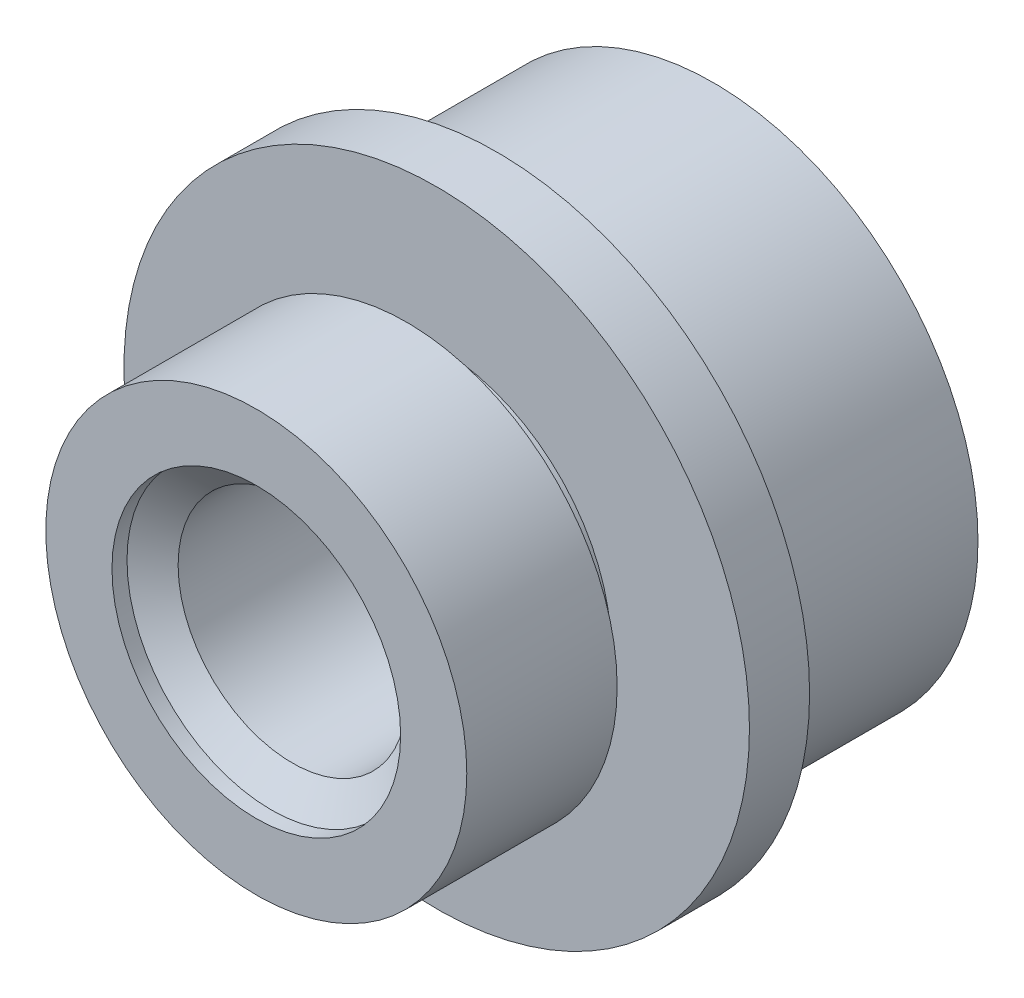
SolidWorks part; units mm, degrees
ref_plane "Front Plane" through (0, 0, 0) normal (0, 0, 1) x (1, 0, 0)
ref_plane "Top Plane" through (0, 0, 0) normal (0, 1, 0) x (1, 0, 0)
ref_plane "Right Plane" through (0, 0, 0) normal (1, 0, 0) x (0, 0, -1)
other "Configuration Table"
sketch "Sketch2" plane through (0, 0, 0) normal (1, 0, 0) x (0, 0, -1)
  line L0 (-28.4925, 0) -> (11.8439, 0) construction
  line L1 (0, 17.5) -> (0, 12)
  line L2 (0, 12) -> (1.25, 12)
  line L3 (1.25, 12) -> (3.0005, 9.5)
  line L4 (3.0005, 9.5) -> (23, 9.5)
  line L5 (23, 9.5) -> (38, 14)
  line L6 (38, 14) -> (38, 22)
  line L7 (38, 22) -> (20, 22)
  line L8 (20, 22) -> (20, 26)
  line L9 (20, 26) -> (15, 26)
  line L10 (15, 26) -> (15, 14.5)
  line L11 (15, 14.5) -> (12.5, 14.5)
  line L12 (12.5, 14.5) -> (12.5, 17.5)
  line L13 (12.5, 17.5) -> (0, 17.5)
  dimension "D1" = 35
  dimension "D2" = 52
  dimension "D3" = 44
  dimension "D4" = 19
  dimension "D5" = 24
  dimension "D6" = 55
  dimension "D7" = 1.25
  dimension "D8" = 2.5
  dimension "D9" = 3
  dimension "D10" = 5
  dimension "D11" = 15
  dimension "D12" = 38
  dimension "D13" = 15
  dimension "D14" = 28
revolve "Revolve1" add sketch "Sketch2" angle 360 about L0
cosmetic thread "Cosmetic Thread1"
